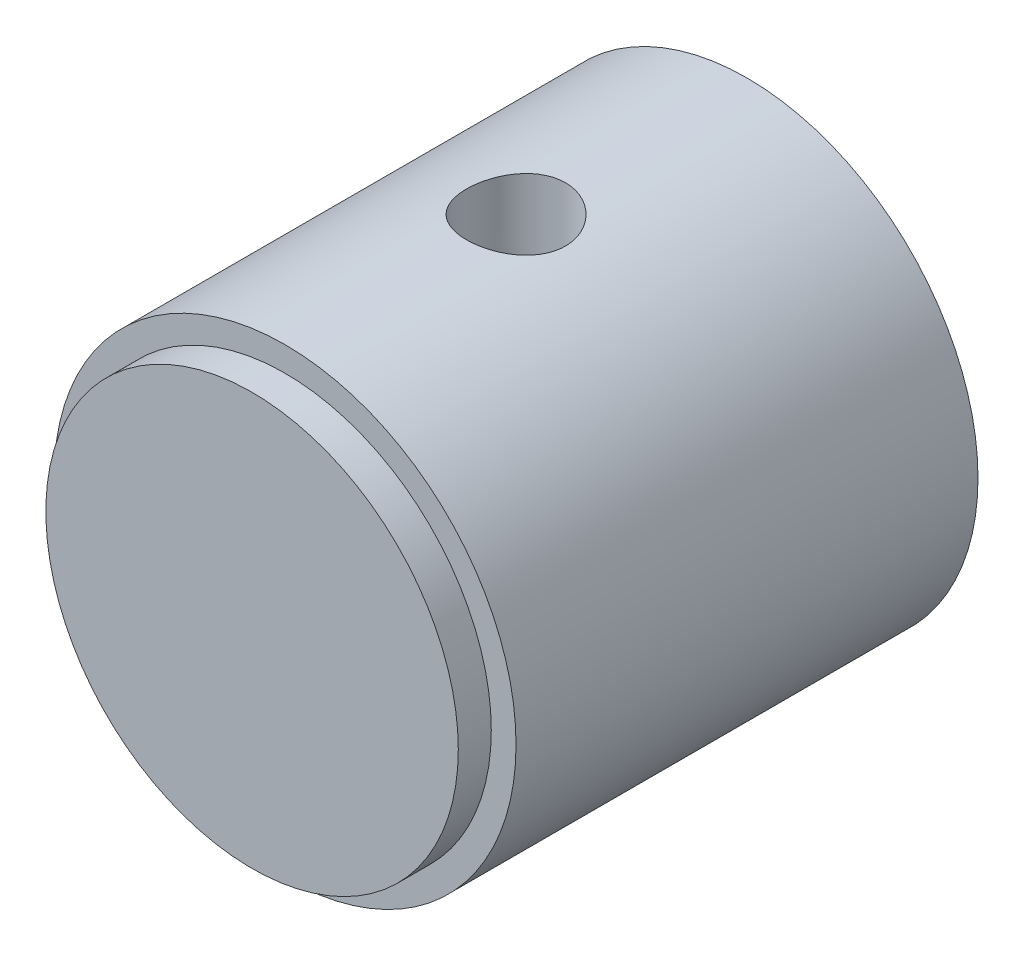
SolidWorks part; units mm, degrees
ref_plane "Front Plane" through (0, 0, 0) normal (0, 0, 1) x (1, 0, 0)
ref_plane "Top Plane" through (0, 0, 0) normal (0, 1, 0) x (1, 0, 0)
ref_plane "Right Plane" through (0, 0, 0) normal (1, 0, 0) x (0, 0, -1)
other "Configuration Table"
sketch "Sketch1" plane through (0, 0, 0) normal (0, 0, 1) x (1, 0, 0)
  circle A0 centre (0, 0) radius 7
  dimension "D1" = 14
extrude "Boss-Extrude1" add sketch "Sketch1" along normal blind 15
sketch "Sketch2" plane through (0, 0, 15) normal (0, 0, 1) x (1, 0, 0)
  circle A0 centre (0, 0) radius 6.25
  circle A1 centre (0, 0) radius 7 construction
  circle A2 centre (0, 0) radius 7
  dimension "D1" = 12.5
extrude "Cut-Extrude1" cut sketch "Sketch2" against normal blind 1
hole_wizard "Ø9.5 (9.5) Diameter Hole1" positions "3DSketch1" profile "Sketch3" hole size "Ø9.5" standard "GB"
sketch3d "3DSketch1"
  point P14 (0, 0, 0)
sketch "Sketch3" plane through (0, 0, 0) normal (1, 0, 0) x (0, 1, 0)
  line L0 (0, 0) -> (0, 13.8541)
  line L1 (0, 13.8541) -> (4.75, 11)
  line L2 (4.75, 11) -> (4.75, 0)
  line L5 (4.75, 0) -> (0, 0)
  line L10 (0, 13.8541) -> (-4.75, 11) construction
  line L11 (0, -6.35) -> (0, 107.95) construction
  dimension "孔直径" = 9.5
  dimension "孔深度" = 11
  dimension "导头角度" = 118
sketch "Sketch4" plane through (0, 0, 0) normal (0, 0, -1) x (-1, 0, 0)
  circle A0 centre (0, 0) radius 6.2
  dimension "D1" = 12.4
extrude "Cut-Extrude2" cut sketch "Sketch4" against normal blind 5 draft 20
sketch "Sketch5" plane through (0, 0, 0) normal (0, 1, 0) x (1, 0, 0)
  line L0 (6.2, 0) -> (-6.2, 0) construction
  circle A0 centre (0, -7) radius 1.5
  dimension "D1" = 3
  dimension "D2" = 7
extrude "Cut-Extrude3" cut sketch "Sketch5" against normal mid plane 20
